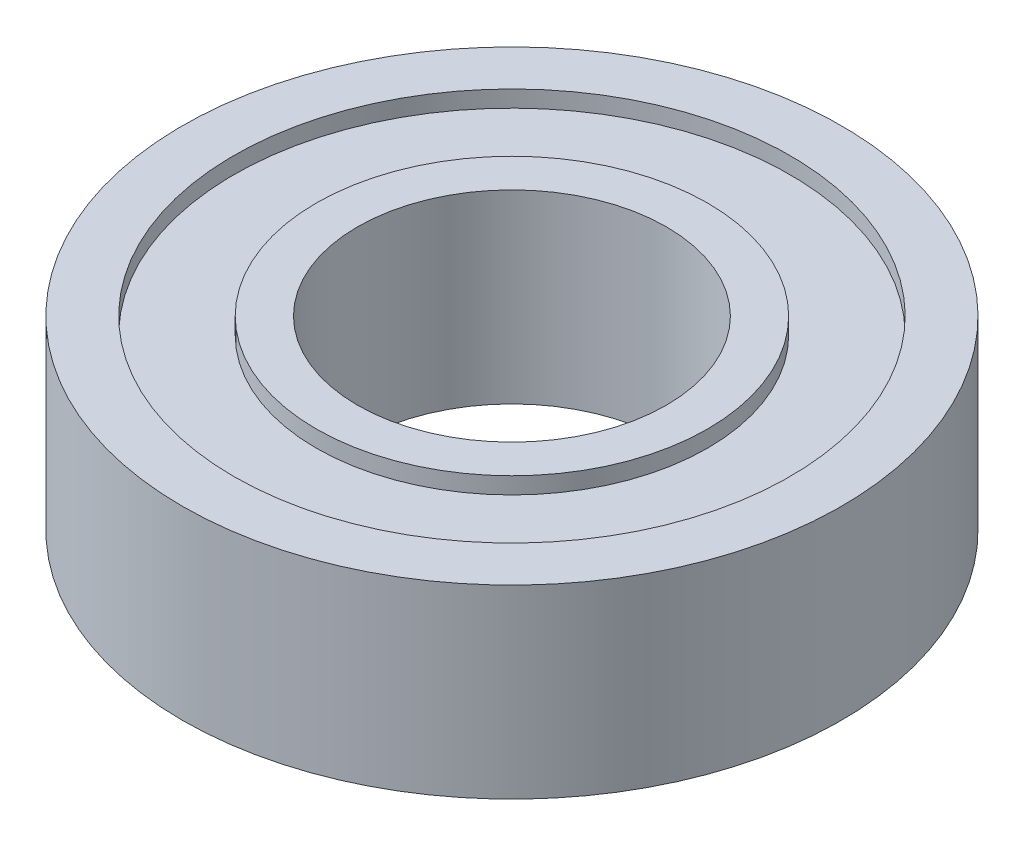
from build123d import *


with BuildPart() as part:
    # 草图1 → 旋转1 (revolve)
    with BuildSketch(Plane.XY, mode=Mode.PRIVATE) as revolve_1_sk:
        Polygon((7.5, 0), (7.5, -9), (9.5, -9), (9.5, -8), (13.5, -8), (13.5, -9), (16, -9), (16, 0), (13.5, 0), (13.5, -0.807209449), (9.5, -0.807209449), (9.5, 0), align=None)
    revolve(revolve_1_sk.sketch.rotate(Axis((0, 13.438321286, 0), (0, -1, 0)), 90), axis=Axis((0, 13.438321286, 0), (0, -1, 0)))


solid = part.part
